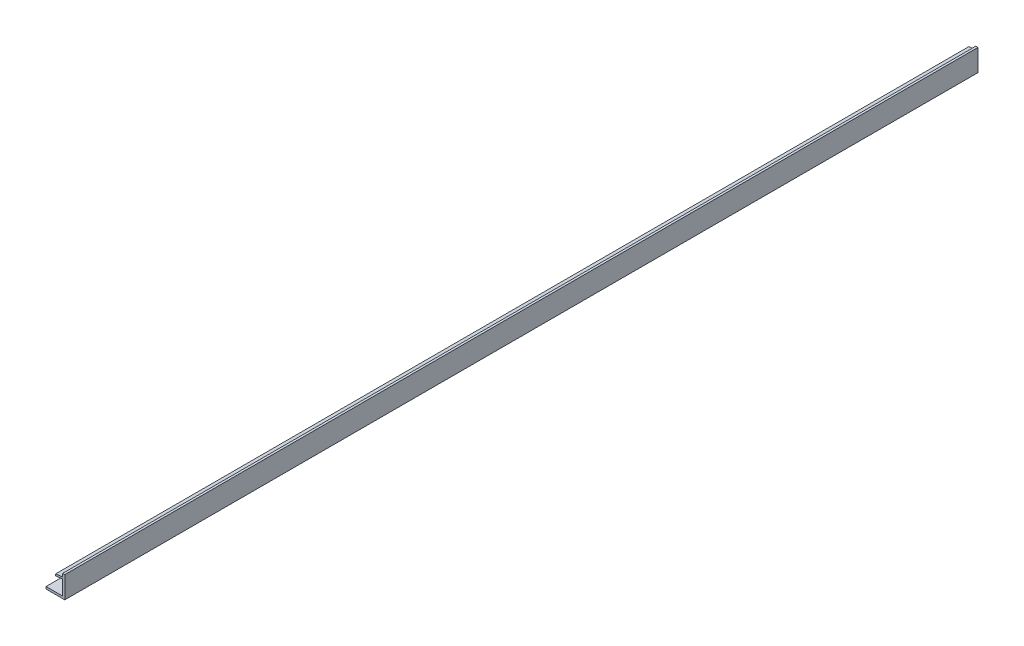
from build123d import *

# Parameters (mm, degrees)
EXTRUDE_1_DEPTH = 1045
EXTRUDE_2_DEPTH = 1045


with BuildPart() as part:
    # 草图1 → 凸台-拉伸1 (new, symmetric)
    with BuildSketch(Plane.XY):
        Polygon((-43, 0), (0, 0), (0, 50), (-5, 50), (-5, 5), (-43, 5), align=None)
    extrude(amount=EXTRUDE_1_DEPTH, both=True)


with BuildPart() as body_2:
    # 草图2 → 凸台-拉伸2 (new, symmetric)
    with BuildSketch(Plane.XY):
        Polygon((-5, 43.031128874), (-21, 41.031128874), (-21, 37), (-5, 39), align=None)
    extrude(amount=EXTRUDE_2_DEPTH, both=True)


solid = Compound([part.part, body_2.part])
